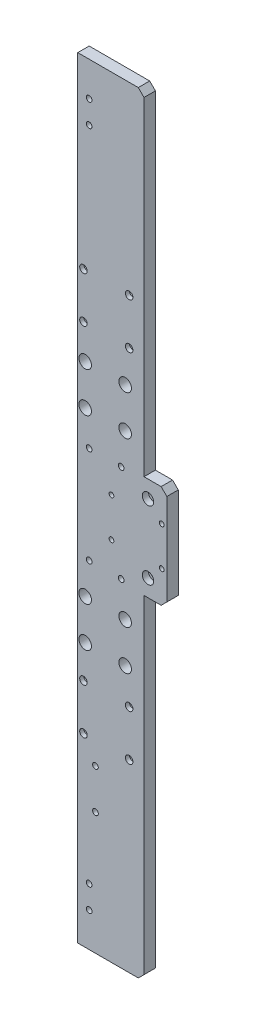
SolidWorks part; units mm, degrees
material "6061-T6"
ref_plane "前视基准面" through (0, 0, 0) normal (0, 0, 1) x (1, 0, 0)
ref_plane "上视基准面" through (0, 0, 0) normal (0, 1, 0) x (1, 0, 0)
ref_plane "右视基准面" through (0, 0, 0) normal (1, 0, 0) x (0, 0, -1)
sketch "草图1" plane through (0, 0, 0) normal (0, 0, 1) x (1, 0, 0)
  line L1 (108, 675) -> (0, 675)
  line L2 (108, 675) -> (108, 0)
  line L3 (108, 0) -> (0, 0)
  line L4 (0, 675) -> (0, 0)
  dimension "D1" = 675
  dimension "D2" = 108
extrude "凸台-拉伸1" add sketch "草图1" along normal blind 10
hole_wizard "M6 螺纹孔1" positions "草图2" profile "草图3" tap size "M6" standard "ISO" end condition through all
sketch "草图2" plane through (0, 0, 10) normal (0, 0, 1) x (1, 0, 0)
  line L0 (0, 337.5) -> (151.089, 337.5) construction
  line L1 (0, 675) -> (0, 0) construction
  line L3 (10, 30) -> (10, 50) construction
  line L5 (0, 0) -> (108, 0) construction
  point P0 (10, 645)
  point P2 (10, 625)
  point P13 (10, 50)
  point P14 (10, 30)
  dimension "D1" = 10
  dimension "D2" = 20
  dimension "D3" = 30
sketch "草图3" plane through (10, 645, 10) normal (1, 0, 0) x (0, -1, 0)
  line L0 (0, 0) -> (0, 10)
  line L1 (0, 10) -> (2.5, 10)
  line L2 (2.5, 10) -> (2.5, 0)
  line L5 (2.5, 0) -> (0, 0)
  line L11 (0, -6.35) -> (0, 107.95) construction
  dimension "通孔螺纹孔钻头直径" = 5
  dimension "通孔螺纹孔钻头深度" = 10
cosmetic thread "孔螺蚊线1" parameters "D2"=6
cosmetic thread "孔螺蚊线2" parameters "D2"=6
cosmetic thread "孔螺蚊线3" parameters "D2"=6
cosmetic thread "孔螺蚊线4" parameters "D2"=6
hole_wizard "M6 六角凹头螺钉的柱形沉头孔1" positions "草图4" profile "草图5" counterbore size "M6" standard "ISO" end condition through all
sketch "草图4" plane through (0, 0, 0) normal (0, 0, -1) x (-1, 0, 0)
  line L0 (0, 337.5) -> (27.2492, 337.5) construction
  line L1 (0, 675) -> (0, 0) construction
  line L3 (-45, 161.5) -> (-5, 161.5) construction
  line L4 (-5, 161.5) -> (-5, 201.5) construction
  line L5 (-5, 201.5) -> (-45, 201.5) construction
  line L6 (-45, 201.5) -> (-45, 161.5) construction
  line L8 (-5, 201.5) -> (-5, 473.5) construction
  line L9 (-5, 473.5) -> (-5, 513.5) construction
  line L10 (-5, 513.5) -> (-45, 513.5) construction
  line L11 (-45, 513.5) -> (-45, 473.5) construction
  line L12 (-45, 473.5) -> (-5, 473.5) construction
  point P0 (-45, 513.5)
  point P2 (-5, 513.5)
  point P4 (-45, 473.5)
  point P6 (-5, 473.5)
  point P15 (-5, 201.5)
  point P16 (-45, 201.5)
  point P17 (-5, 161.5)
  point P18 (-45, 161.5)
  point P37 (-5, 181.5)
  dimension "D1" = 272
  dimension "D2" = 5
  dimension "D3" = 40
  dimension "D4" = 40
sketch "草图5" plane through (45, 513.5, 0) normal (1, 0, 0) x (0, 1, 0)
  line L0 (0, 0) -> (0, 10)
  line L1 (0, 10) -> (3.3, 10)
  line L3 (3.3, 10) -> (3.3, 6.4)
  line L4 (3.3, 6.4) -> (5.5, 6.4)
  line L5 (5.5, 6.4) -> (5.5, 0)
  line L7 (5.5, 0) -> (0, 0)
  line L11 (0, -6.35) -> (0, 107.95) construction
  dimension "通孔孔直径" = 6.6
  dimension "通孔孔深度" = 10
  dimension "柱形沉头孔直径" = 11
  dimension "柱形沉头孔深度" = 6.4
hole_wizard "M5 螺纹孔1" positions "草图6" profile "草图7" tap size "M5" standard "ISO"
sketch "草图6" plane through (0, 0, 10) normal (0, 0, 1) x (1, 0, 0)
  line L0 (29.5, 320.5) -> (73.5, 320.5) construction
  line L1 (73.5, 320.5) -> (73.5, 354.5) construction
  line L2 (73.5, 354.5) -> (29.5, 354.5) construction
  line L3 (29.5, 354.5) -> (29.5, 320.5) construction
  line L5 (29.5, 337.5) -> (0, 337.5) construction
  line L6 (0, 675) -> (0, 0) construction
  point P0 (29.5, 354.5)
  point P2 (73.5, 354.5)
  point P4 (29.5, 320.5)
  point P6 (73.5, 320.5)
  dimension "D1" = 29.5
  dimension "D2" = 44
  dimension "D3" = 34
sketch "草图7" plane through (29.5, 354.5, 10) normal (1, 0, 0) x (0, -1, 0)
  line L0 (0, 0) -> (0, 15.2618)
  line L1 (0, 15.2618) -> (2.1, 14)
  line L2 (2.1, 14) -> (2.1, 0)
  line L5 (2.1, 0) -> (0, 0)
  line L10 (0, 15.2618) -> (-2.1, 14) construction
  line L11 (0, -6.35) -> (0, 107.95) construction
  dimension "螺纹孔钻头直径" = 4.2
  dimension "螺纹孔钻头深度" = 14
  dimension "导头角度" = 118
cosmetic thread "孔螺蚊线6" parameters "D1"=10, "D2"=5
cosmetic thread "孔螺蚊线8" parameters "D1"=10, "D2"=5
cosmetic thread "孔螺蚊线17" parameters "D1"=10, "D2"=5
cosmetic thread "孔螺蚊线18" parameters "D1"=10, "D2"=5
hole_wizard "M6 螺纹孔2" positions "草图8" profile "草图9" tap size "M6" standard "ISO"
sketch "草图8" plane through (0, 0, 10) normal (0, 0, 1) x (1, 0, 0)
  line L0 (97.5, 396.5) -> (97.5, 431.5) construction
  line L2 (108, 0) -> (108, 675) construction
  line L3 (108, 337.5) -> (132.6323, 337.5) construction
  point P0 (97.5, 431.5)
  point P2 (97.5, 396.5)
  dimension "D1" = 10.5
  dimension "D2" = 35
  dimension "D3" = 59
sketch "草图9" plane through (97.5, 431.5, 10) normal (1, 0, 0) x (0, -1, 0)
  line L0 (0, 0) -> (0, 18.5022)
  line L1 (0, 18.5022) -> (2.5, 17)
  line L2 (2.5, 17) -> (2.5, 0)
  line L5 (2.5, 0) -> (0, 0)
  line L10 (0, 18.5022) -> (-2.5, 17) construction
  line L11 (0, -6.35) -> (0, 107.95) construction
  dimension "螺纹孔钻头直径" = 5
  dimension "螺纹孔钻头深度" = 17
  dimension "导头角度" = 118
cosmetic thread "孔螺蚊线9" parameters "D1"=10, "D2"=6
cosmetic thread "孔螺蚊线10" parameters "D1"=10, "D2"=6
hole_wizard "M5 六角凹头螺钉的柱形沉头孔1" positions "草图10" profile "草图11" counterbore size "M5" standard "ISO"
sketch "草图10" plane through (0, 0, 10) normal (0, 0, 1) x (1, 0, 0)
  line L0 (91.5, 367.5) -> (61.5, 367.5) construction
  line L1 (61.5, 367.5) -> (61.5, 307.5) construction
  line L2 (61.5, 307.5) -> (91.5, 307.5) construction
  line L3 (91.5, 307.5) -> (91.5, 367.5) construction
  line L5 (91.5, 337.5) -> (108, 337.5) construction
  line L6 (108, 0) -> (108, 675) construction
  point P0 (61.5, 367.5)
  point P2 (91.5, 367.5)
  point P4 (61.5, 307.5)
  point P6 (91.5, 307.5)
  dimension "D1" = 16.5
  dimension "D2" = 30
  dimension "D3" = 60
sketch "草图11" plane through (61.5, 367.5, 10) normal (1, 0, 0) x (0, -1, 0)
  line L0 (0, 0) -> (0, 15.6524)
  line L1 (0, 15.6524) -> (2.75, 14)
  line L2 (2.75, 14) -> (2.75, 5.4)
  line L3 (2.75, 5.4) -> (5, 5.4)
  line L4 (5, 5.4) -> (5, 0)
  line L5 (5, 0) -> (0, 0)
  line L10 (0, 15.6524) -> (-2.75, 14) construction
  line L11 (0, -6.35) -> (0, 107.95) construction
  dimension "孔直径" = 5.5
  dimension "孔深度" = 14
  dimension "柱形沉头孔直径" = 10
  dimension "柱形沉头孔深度" = 5.4
  dimension "导头角度" = 118
hole_wizard "M6 螺纹孔3" positions "草图12" profile "草图13" tap size "M6" standard "ISO"
sketch "草图12" plane through (0, 0, 0) normal (0, 0, -1) x (-1, 0, 0)
  line L0 (-38, 295) -> (-10, 295) construction
  line L1 (-10, 295) -> (-10, 380) construction
  line L2 (-10, 380) -> (-38, 380) construction
  line L3 (-38, 380) -> (-38, 295) construction
  line L5 (-10, 337.5) -> (0, 337.5) construction
  line L6 (0, 471.2087) -> (0, 203.7913) construction
  point P0 (-38, 380)
  point P2 (-10, 380)
  point P4 (-38, 295)
  point P6 (-10, 295)
  dimension "D1" = 10
  dimension "D2" = 85
  dimension "D3" = 28
sketch "草图13" plane through (38, 380, 0) normal (1, 0, 0) x (0, 1, 0)
  line L0 (0, 0) -> (0, 18.5022)
  line L1 (0, 18.5022) -> (2.5, 17)
  line L2 (2.5, 17) -> (2.5, 0)
  line L5 (2.5, 0) -> (0, 0)
  line L10 (0, 18.5022) -> (-2.5, 17) construction
  line L11 (0, -6.35) -> (0, 107.95) construction
  dimension "螺纹孔钻头直径" = 5
  dimension "螺纹孔钻头深度" = 17
  dimension "导头角度" = 118
cosmetic thread "孔螺蚊线11" parameters "D1"=10, "D2"=6
cosmetic thread "孔螺蚊线12" parameters "D1"=10, "D2"=6
cosmetic thread "孔螺蚊线13" parameters "D1"=10, "D2"=6
cosmetic thread "孔螺蚊线14" parameters "D1"=10, "D2"=6
sketch "草图14" plane through (0, 0, 10) normal (0, 0, 1) x (1, 0, 0)
  line L0 (6.5, 266) -> (6.5, 409) construction
  line L1 (6.5, 409) -> (41.5, 409) construction
  line L2 (41.5, 409) -> (41.5, 266) construction
  line L3 (41.5, 266) -> (41.5, 231) construction
  line L4 (41.5, 231) -> (6.5, 231) construction
  line L5 (6.5, 231) -> (6.5, 266) construction
  line L6 (6.5, 266) -> (41.5, 266) construction
  line L7 (6.5, 409) -> (6.5, 444) construction
  line L8 (6.5, 444) -> (41.5, 444) construction
  line L9 (41.5, 444) -> (41.5, 409) construction
  line L10 (41.5, 337.5) -> (108, 337.5) construction
  line L11 (108, 0) -> (108, 675) construction
  circle A0 centre (41.5, 444) radius 5.5
  circle A1 centre (6.5, 444) radius 5.5
  circle A2 centre (41.5, 409) radius 5.5
  circle A3 centre (6.5, 409) radius 5.5
  circle A4 centre (41.5, 266) radius 5.5
  circle A5 centre (41.5, 231) radius 5.5
  circle A6 centre (6.5, 231) radius 5.5
  circle A7 centre (6.5, 266) radius 5.5
  dimension "D6" = 11
  dimension "D1" = 35
  dimension "D2" = 35
  dimension "D3" = 143
  dimension "D4" = 35
  dimension "D5" = 66.5
extrude "切除-拉伸1" cut sketch "草图14" against normal blind 60
sketch "草图15" plane through (0, 0, 10) normal (0, 0, 1) x (1, 0, 0)
  line L5 (78, 337.5) -> (0, 337.5) construction
  line L6 (108, 675) -> (58, 675)
  line L7 (108, 675) -> (108, 382.5)
  line L8 (108, 382.5) -> (58, 382.5)
  line L9 (58, 675) -> (58, 382.5)
  line L10 (108, 0) -> (58, 0)
  line L11 (108, 0) -> (108, 292.5)
  line L12 (108, 292.5) -> (58, 292.5)
  line L13 (58, 0) -> (58, 292.5)
  line L14 (78, 382.5) -> (108, 382.5)
  line L15 (78, 382.5) -> (78, 292.5)
  line L16 (78, 292.5) -> (108, 292.5)
  line L17 (108, 382.5) -> (108, 292.5)
  line L18 (0, 675) -> (0, 0) construction
  line L19 (58, 292.5) -> (58, 382.5) construction
  circle M18 centre (91.5, 367.5) radius 5
  circle M20 centre (91.5, 307.5) radius 5
  circle M21 centre (97.5, 431.5) radius 2.5
  circle M22 centre (97.5, 396.5) radius 2.5
  line M39 (108, 0) -> (108, 675)
  line M40 (108, 675) -> (0, 675)
  line M42 (0, 0) -> (108, 0)
  dimension "D1" = 50
  dimension "D2" = 90
  dimension "D3" = 30
extrude "切除-拉伸2" cut sketch "草图15" against normal through all contours L9 L8 M40 M39 M21 M22 | L8 L15 L12 M39 M20 M18 | L13 L12 M42 M39 | M18 | M20
chamfer "倒角1" distance 5 angle 45 4 edges at (58, 675, 5) (78, 382.5, 5) (78, 292.5, 5) (58, 0, 5)
hole_wizard "M6 螺纹孔4" positions "草图16" profile "草图17" tap size "M6" standard "ISO" end condition through all
sketch "草图16" plane through (0, 0, 10) normal (0, 0, 1) x (1, 0, 0)
  line L0 (15.5, 107) -> (15.5, 142) construction
  line L2 (0, 675) -> (0, 0) construction
  line L3 (0, 0) -> (53, 0) construction
  point P0 (15.5, 142)
  point P2 (15.5, 107)
  dimension "D1" = 15.5
  dimension "D2" = 107
  dimension "D3" = 35
sketch "草图17" plane through (15.5, 142, 10) normal (1, 0, 0) x (0, -1, 0)
  line L0 (0, 0) -> (0, 10)
  line L1 (0, 10) -> (2.5, 10)
  line L2 (2.5, 10) -> (2.5, 0)
  line L5 (2.5, 0) -> (0, 0)
  line L11 (0, -6.35) -> (0, 107.95) construction
  dimension "通孔螺纹孔钻头直径" = 5
  dimension "通孔螺纹孔钻头深度" = 10
cosmetic thread "孔螺蚊线15" parameters "D2"=6
cosmetic thread "孔螺蚊线16" parameters "D2"=6
